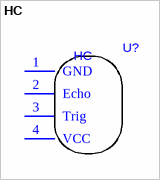
[diagram p0: symbol HC]
# Altium schematic symbol library MISC84237-14.SchLib: 1 symbol
Pins are listed as number, name and electrical type; pins without a type are passive.


## HC
designator U?
footprint HC-SR04
pins: 1 GND, 2 Echo, 3 Trig, 4 VCC